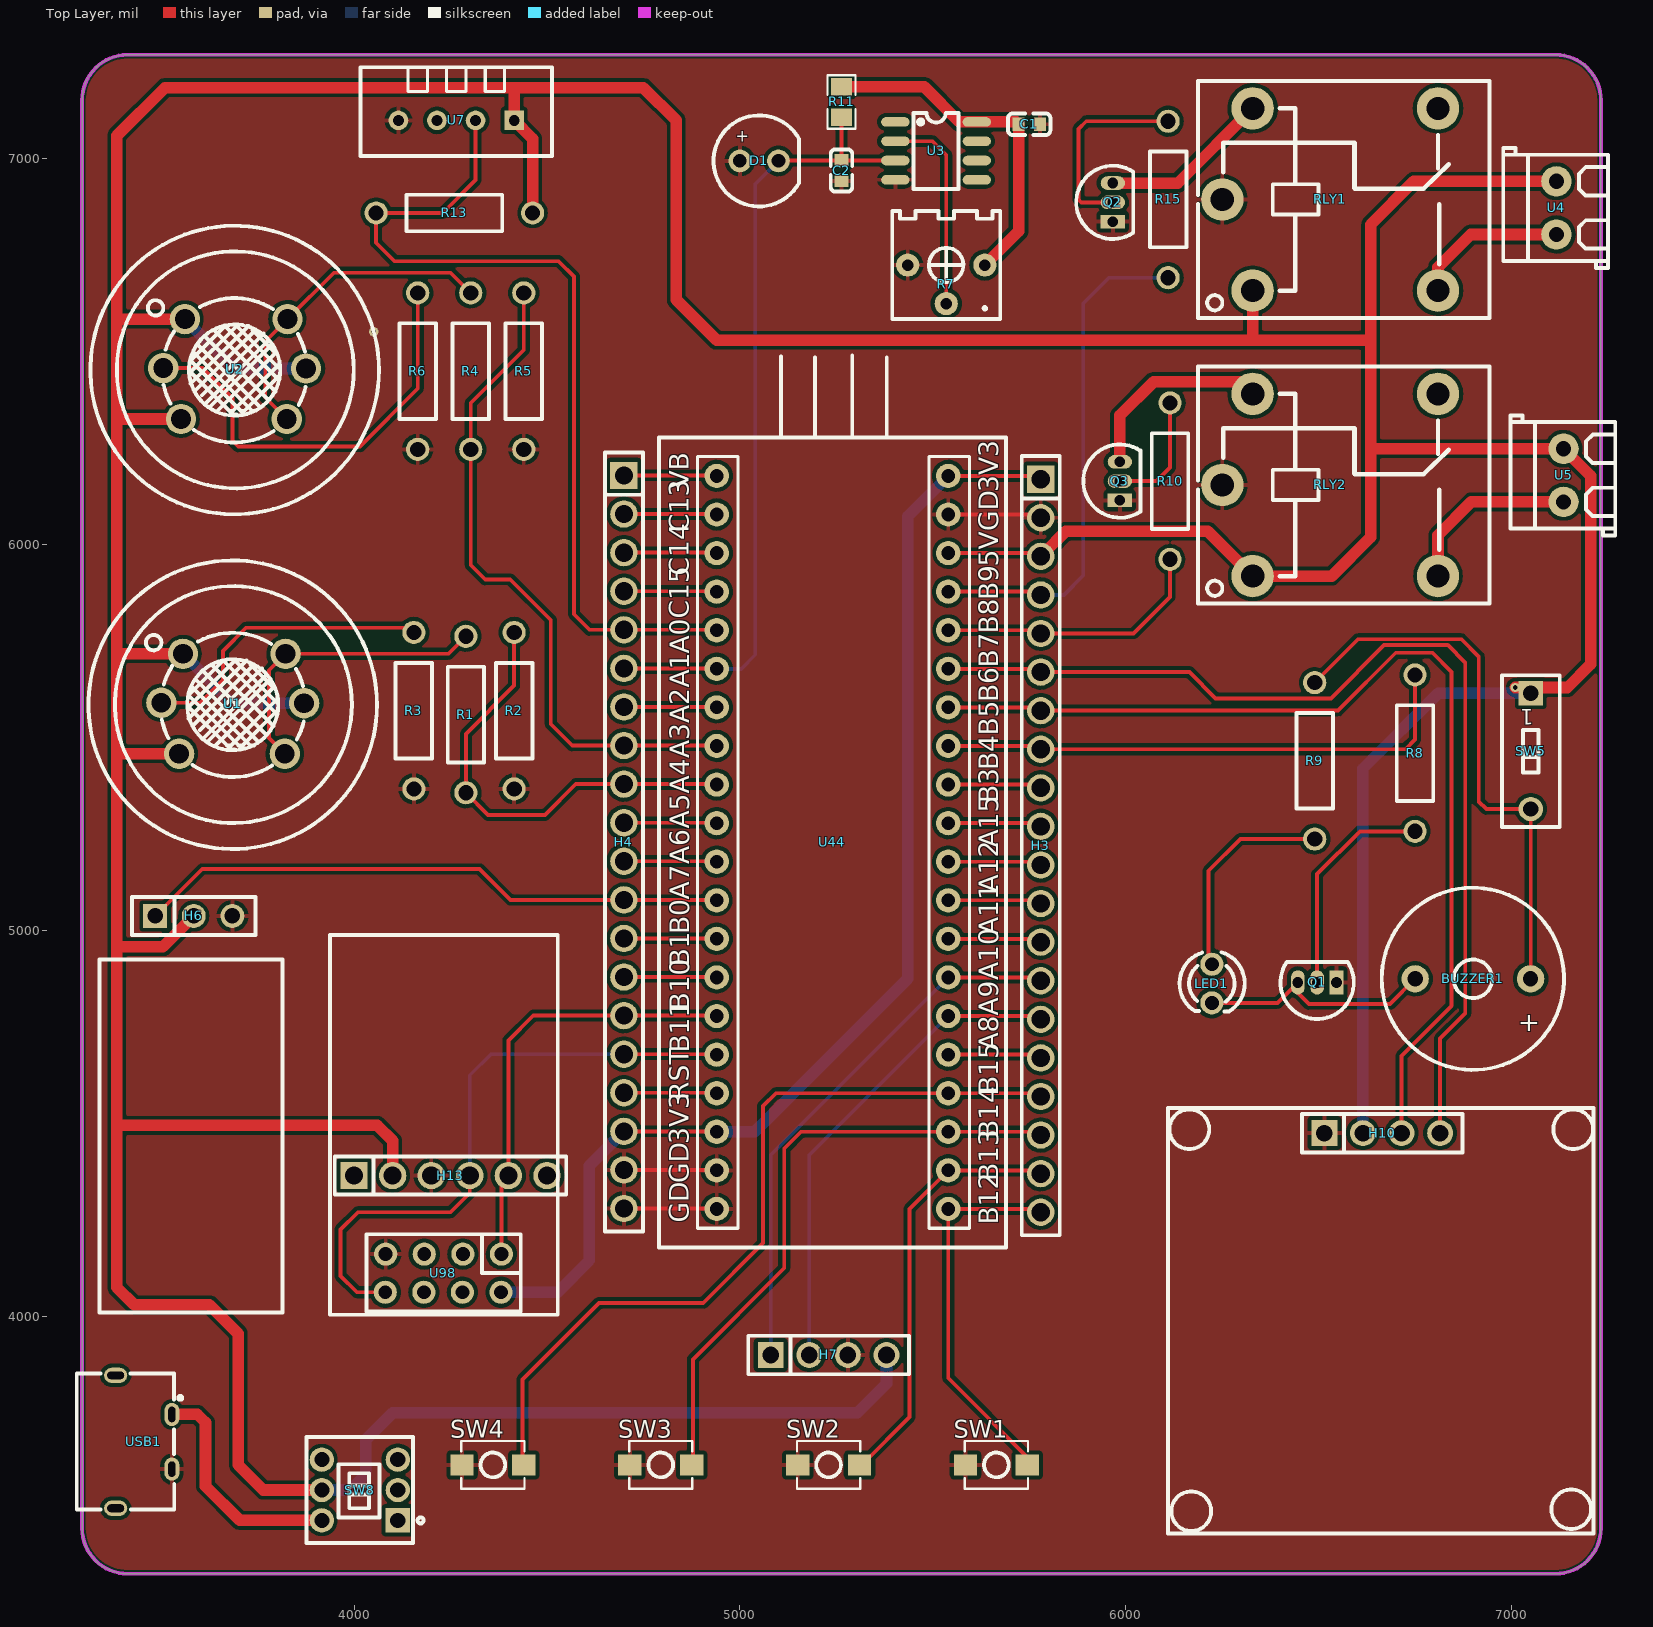
[diagram p0: Top Layer view]
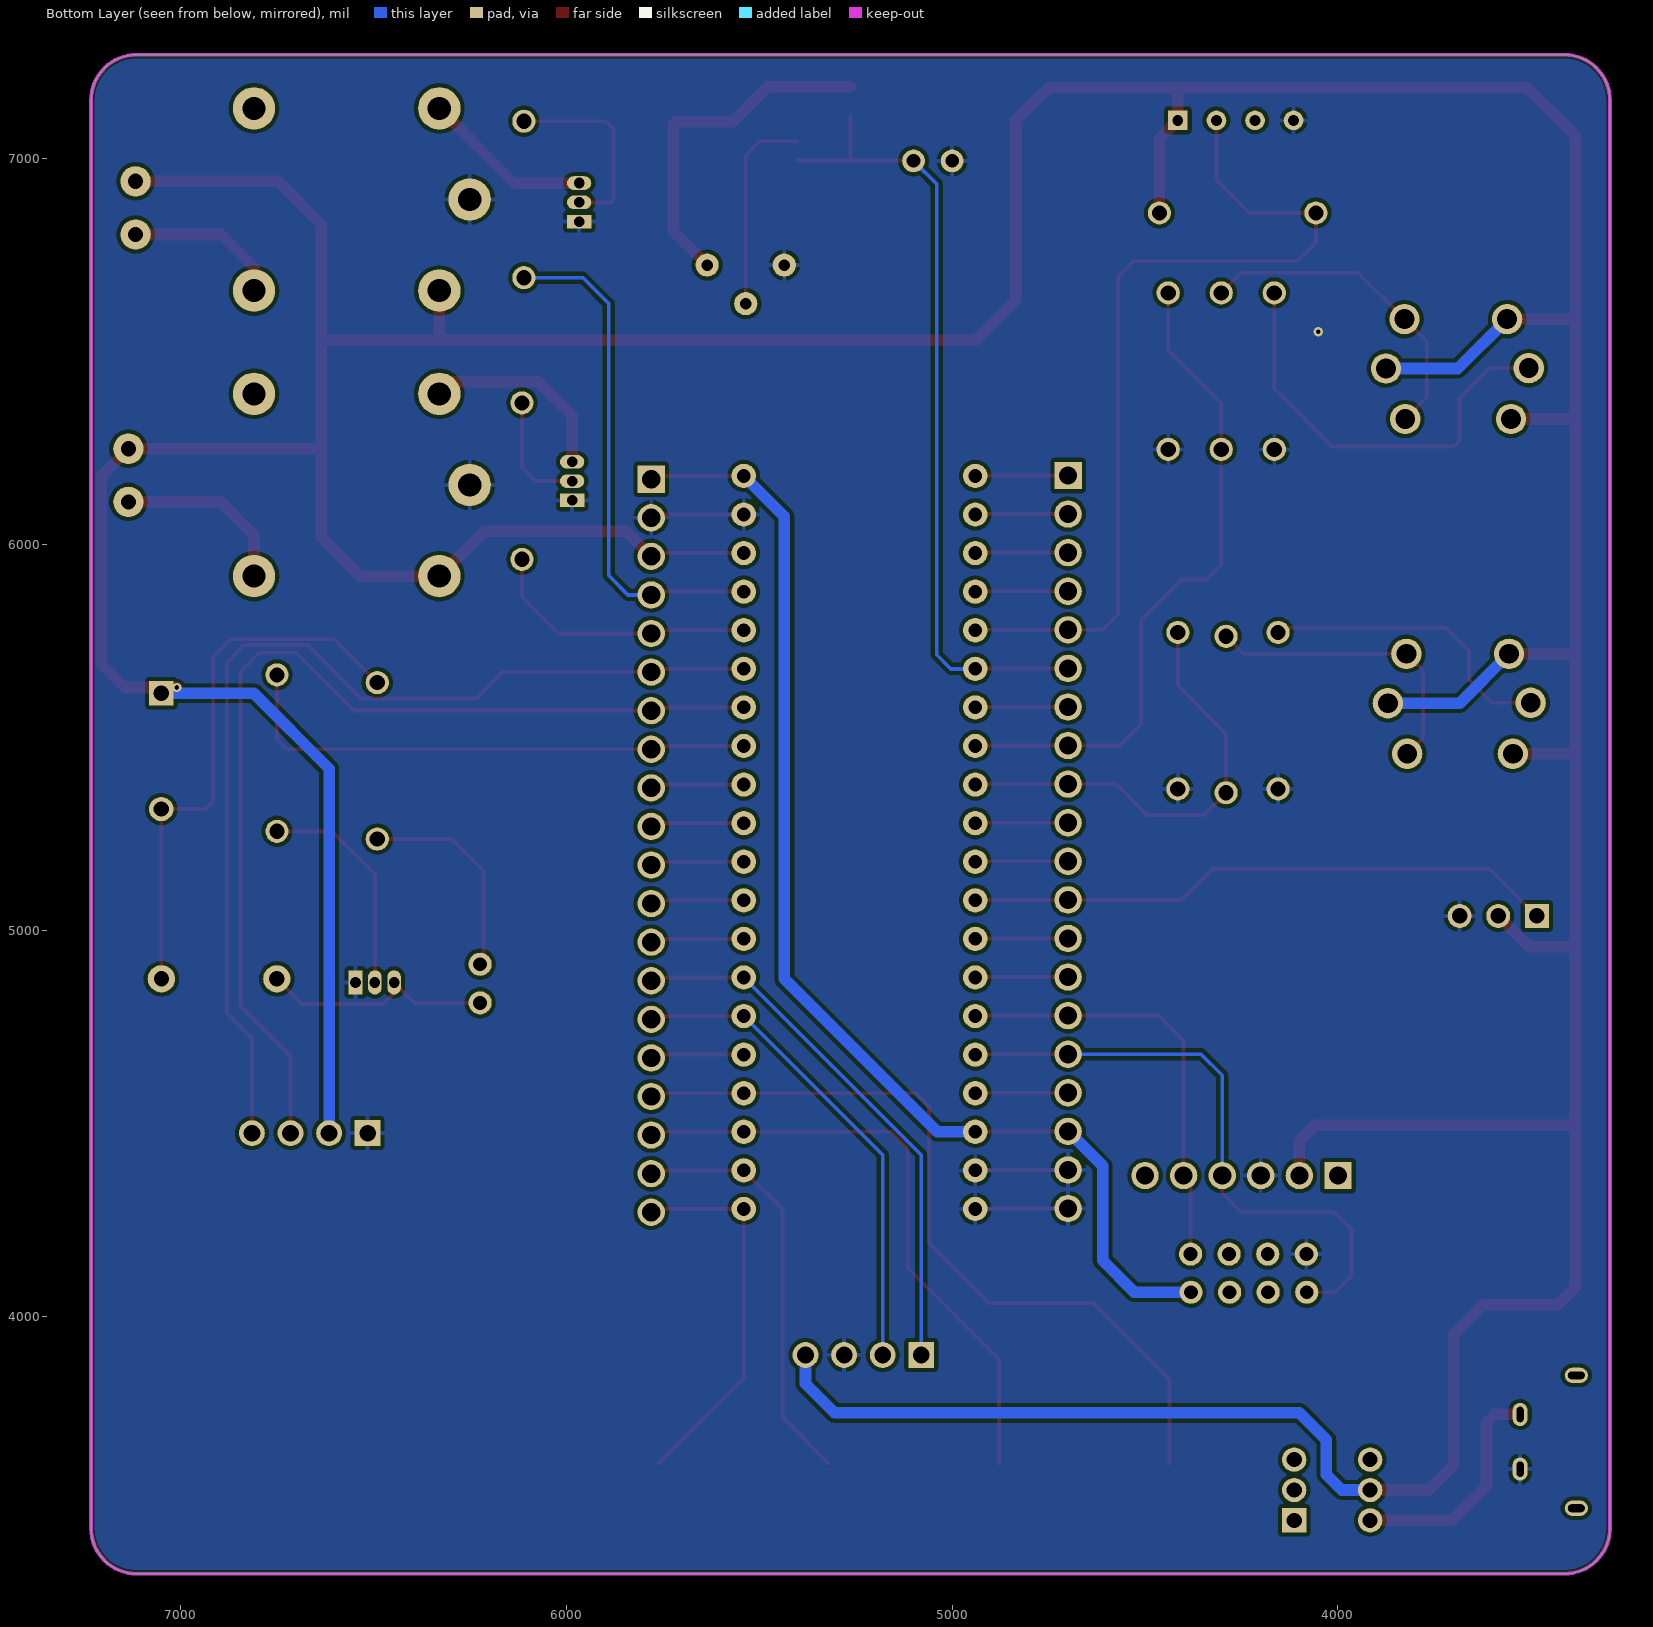
[diagram p1: Bottom Layer view, seen from below]
# Altium PCB MISC52003.pcbdoc
Units mil, origin at the board's own origin, x right, y up, seen from the top; angles counter-clockwise.
Board outline 3937.01 x 3937.01 mil, 2 copper layers (Top Layer, Bottom Layer), stack 62.206 mil thick; 44 components, 55 nets, 209 pads, 2 vias.

## Layer stack, top to bottom
Top Solder Mask Layer: solder mask 0.394, Dk 3.3
Top Layer: signal copper 1.379
Dielectric1: surface 59.449, FR4, Dk 4.5
Bottom Layer: signal copper 1.378
Bottom Solder Mask Layer: solder mask 0.394, Dk 3.3

## Board outline
3413.11,7270 ccw(c3413.11,7151.89) 3295,7151.89 3295,3451.1 ccw(c3413.11,3451.1) 3413.11,3332.99 7113.9,3332.99 ccw(c7113.9,3451.1) 7232.01,3451.1 7232.01,7151.89 ccw(c7113.9,7151.89) 7113.9,7270

## Design rules (kind name [scope] priority, off if disabled: settings)
BoardOutlineClearance copperThickness2oz_1 [All] p2 off: genericclearance=7.99 ignorepadtopadclearanceinfootprint=FALSE except(0: Arc-SplitContinuation Track-SplitContinuation SMDPad-SplitContinuation THPad-SplitContinuation Via-SplitContinuation Fill-SplitContinuation Region-SplitContinuation Poly-SplitContinuation Text-SplitContinuation Hole-SplitContinuation; 5.98: Arc-CutoutEdge SMDPad-CutoutEdge THPad-CutoutEdge Via-CutoutEdge Fill-CutoutEdge Region-CutoutEdge Text-CutoutEdge; 6.93: Hole-OutlineEdge Hole-CutoutEdge; 10: Poly-OutlineEdge Poly-CutoutEdge; 11.81: Arc-OutlineEdge Track-OutlineEdge SMDPad-OutlineEdge THPad-OutlineEdge Via-OutlineEdge Fill-OutlineEdge Region-OutlineEdge Text-OutlineEdge Track-CutoutEdge)
BoardOutlineClearance copperThickness1oz_1 [All] p4: genericclearance=4.02 ignorepadtopadclearanceinfootprint=FALSE except(0: Arc-SplitContinuation Track-SplitContinuation SMDPad-SplitContinuation THPad-SplitContinuation Via-SplitContinuation Fill-SplitContinuation Region-SplitContinuation Poly-SplitContinuation Text-SplitContinuation Hole-SplitContinuation; 6: SMDPad-CutoutEdge THPad-CutoutEdge Via-CutoutEdge Fill-CutoutEdge Region-CutoutEdge Text-CutoutEdge; 6.93: Hole-OutlineEdge Hole-CutoutEdge; 10: Poly-OutlineEdge Poly-CutoutEdge; 11.8: Arc-OutlineEdge Track-OutlineEdge SMDPad-OutlineEdge THPad-OutlineEdge Via-OutlineEdge Fill-OutlineEdge Region-OutlineEdge Text-OutlineEdge; 11.81: Arc-CutoutEdge Track-CutoutEdge)
Clearance copperThickness2oz [All] p1 off: gap=7.99 ignorepadtopadclearanceinfootprint=FALSE except(5.98: SMDPad-Track SMDPad-SMDPad THPad-Track SMDPad-THPad THPad-THPad Track-Via SMDPad-Via THPad-Via Via-Via Fill-Track Region-Track Fill-SMDPad Region-SMDPad Fill-THPad Region-THPad Fill-Via Region-Via Fill-Fill Fill-Region Region-Region Arc-Track Arc-SMDPad Arc-THPad Arc-Via Fill-Arc Region-Arc Arc-Arc Text-Track SMDPad-Text Text-THPad Text-Via Fill-Text Region-Text Arc-Text Text-Text; 6.93: Hole-Track Hole-SMDPad Hole-THPad Hole-Via Fill-Hole Region-Hole Hole-Arc Hole-Text; 10: Poly-Track Poly-SMDPad Poly-THPad Poly-Via Poly-Fill Poly-Region Poly-Poly Poly-Arc Poly-Text Poly-Hole)
Clearance copperThickness1oz [All] p3: gap=4.02 ignorepadtopadclearanceinfootprint=FALSE except(5.98: SMDPad-Track SMDPad-SMDPad THPad-Track SMDPad-THPad THPad-THPad Track-Via SMDPad-Via THPad-Via Via-Via Fill-Track Region-Track Fill-SMDPad Region-SMDPad Fill-THPad Region-THPad Fill-Via Region-Via Fill-Fill Fill-Region Region-Region; 6: Arc-Track Arc-SMDPad Arc-THPad Arc-Via Fill-Arc Region-Arc Arc-Arc Text-Track SMDPad-Text Text-THPad Text-Via Fill-Text Region-Text Arc-Text Text-Text; 6.93: Hole-Track Hole-SMDPad Hole-THPad Hole-Via Fill-Hole Region-Hole Hole-Arc Hole-Text; 10: Poly-Track Poly-SMDPad Poly-THPad Poly-Via Poly-Fill Poly-Region Poly-Poly Poly-Arc Poly-Text Poly-Hole)
Creepage creepage [All] p1: checkdistance=0 ignoreinternallayers=TRUE applytopolygonpour=TRUE
DiffPairsRouting differentialPair [All] p1: maxlimit=6 minlimit=6 mostfreqgap=6 toplayer_minwidth=5 toplayer_prefwidth=10 toplayer_maxwidth=100 toplayer_mingap=6 toplayer_prefgap=6 toplayer_maxgap=6 bottomlayer_minwidth=5 bottomlayer_prefwidth=10 bottomlayer_maxwidth=100 bottomlayer_mingap=6 bottomlayer_prefgap=6 bottomlayer_maxgap=6 maxuncoupledlength=10
HoleToHoleClearance otherClearance [All] p1: gap=11.81 allowstackedmicrovias=TRUE
Length netLength [All] p1: minlimit=0 maxlimit=0
MatchedLengths netLengthTolerance [All] p1: tolerance=1000
PasteMaskExpansion pasteMaskExpansion [All] p1: expansion=0
PlaneConnect innerPlane [All] p1: planeconnectstyle=Relief reliefexpansion=20 reliefentries=4 reliefconductorwidth=10 reliefairgap=10
PolygonConnect copperRegion [(InNet('GND'))] p1: connectstyle=Relief reliefconductorwidth=10 reliefentries=4 polygonreliefangle="90 Angle" airgapwidth=10 via.connectstyle=Relief via.reliefconductorwidth=10 via.reliefentries=4 via.polygonreliefangle="90 Angle" via.airgapwidth=10
RoutingVias viaSize [All] p1: holewidth=12.01 width=24.02 viastyle="Through Hole" minholewidth=11.81 minwidth=19.68 maxholewidth=248.03 maxwidth=393.7
SolderMaskExpansion solderMaskExpansion [IsVia] p1: expansion=-1000 istentingtop=TRUE
SolderMaskExpansion solderMaskExpansion [All] p2: expansion=2 istentingtop=FALSE
Width copperThickness2oz_2 [All] p1 off: maxlimit=100 minlimit=8 preferedwidth=10
Width copperThickness1oz_2 [All] p2: maxlimit=100 minlimit=5 preferedwidth=10

## Components (designator, comment, footprint, x,y, rotation, side; value= is the part's Value field where it differs from the comment)
BUZZER1 "2.3kHz" BUZ-TH_BD12.0-P7.60-D0.6-FD 6900,4875 r180 top
C1 "100nF" C0603 5750,7090 r180 top
C2 "100nF" C0603 5263.49,6970 r90 top
D1 "IR receiver" "IR 接收 D5" 5055,6995 r0 top
H3 "" HDR-TH_20P-P2.54-V-F 5780,5220 r270 top
H4 "" HDR-TH_20P-P2.54-V-F 4699.46,5229.58 r270 top
H6 "" HDR-TH_3P-P2.54-V-F 3584.58,5037.88 r0 top
H7 "" HDR-TH_4P-P2.54-V-F 5230,3900 r0 top
H10 "2.54-1*4P female" HDR-TH_4P-P2.54-V-F 6665,4475 r0 top
H13 "" HDR-TH_6P-P2.54-V-M-1 4250,4365 r0 top
LED1 "" LED_TH-3mm 6223.5,4862.73 r270 top
Q1 "" S8050_TO_92 6496.32,4865.58 r180 top
Q2 "" S8050_TO_92 5966.77,6887.54 r90 top
Q3 "" S8050_TO_92 5985,6165 r90 top
R1 "10kΩ" Res_1/4W 4290,5560 r90 top
R2 "10kΩ" Res_1/4W 4415,5570 r90 top
R3 "5Ω" Res_1/4W 4155,5570 r90 top
R4 "10kΩ" Res_1/4W 4302.5,6450 r90 top
R5 "10kΩ" Res_1/4W 4440,6450 r90 top
R6 "5Ω" Res_1/4W 4165,6450 r90 top
R7 "-" RES-ADJ-TH_3362P 5535,6675 r180 top
R8 "1kΩ" Res_1/4W 6750,5460 r270 top
R9 "120" Res_1/4W 6490,5440 r270 top
R10 "1kΩ" Res_1/4W 6115,6165 r90 top
R11 "10K" R0805 5263.49,7147.68 r90 top
R13 "10kΩ" Res_1/4W 4260,6860 r0 top
R15 "1kΩ" Res_1/4W 6110,6895 r90 top
RLY1 "SRD-05VDC-SL-C" RELAY-TH_SRD-XXVDC-XL-C 6530,6895 r0 top
RLY2 "SRD-05VDC-SL-C" RELAY-TH_SRD-XXVDC-XL-C 6530,6155 r0 top
SW1 "" Key_SMD_3x4x2 5665,3615 r0 top
SW2 "" Key_SMD_3x4x2 5230,3615 r0 top
SW3 "" Key_SMD_3x4x2 4795,3615 r0 top
SW4 "" Key_SMD_3x4x2 4360,3615 r0 top
SW5 "NDS-01V" SW-TH_2P-L3.9-W9.9-P2.54-LS7.6 7050,5465 r270 top
SW8 "TK-6700-1" SW-TH_TK-6700-1 4015,3550 r90 top
U1 "MQ-2" SENSOR-TH_MQ-2 3685.58,5587.88 r0 top
U2 "MQ-5" SENSOR-TH_MQ-2 3690.58,6455.41 r0 top
U3 "LM393" SOP-8_L4.9-W3.9-P1.27-LS6.0-BL 5508.69,7020.94 r270 top
U4 "KF350-3.5-2P" CONN-TH_P3.50_KF350-3.5-2P 7116.51,6873.11 r90 top
U5 "KF350-3.5-2P" CONN-TH_P3.50_KF350-3.5-2P 7135,6180 r90 top
U7 "DHT11" SENSOR-TH_DHT11 4265,7100 r180 top
U44 "" STM32最小系统板 5280,5485 r0 top
U98 "" WiFi封装 4230,4370 r0 top
USB1 "KH-TYPE-C-2P" USB-SMD_KH-TYPE-C-2P 3455,3675 r270 top

## Footprints (in the part's own frame and the unit in brackets; to place one, negate y for a bottom-side part, rotate by r counter-clockwise, add the part's x,y. Pads: shape width x height; smd on the part's side, far side on the other; paste and mask are expansions set on the pad)
BUZ-TH_BD12.0-P7.60-D0.6-FD [mm]
  round 1.8 hole 1 paste+0 mask+0.051: 1(-3.8,0) 2(3.8,0)
  silkscreen extent -6,-6 6,6
C0603 [mm]
  rect 0.8x0.9 smd: 1(-0.7,0) 2(0.7,0)
  silkscreen extent -1.39,-0.71 1.39,0.71
CONN-TH_P3.50_KF350-3.5-2P [mm]
  round 2 hole 1: 1(-1.75,0) 2(1.75,0)
  silkscreen extent -3.95,-3.4 3.95,3.5
HDR-TH_3P-P2.54-V-F [mil]
  rect 62x62 hole 40.16: 1(-100,0)
  round 62 hole 40.16: 2(0,0) 3(100,0)
  silkscreen extent -160,-49 160,49
HDR-TH_4P-P2.54-V-F [mm]
  rect 1.7x1.7 hole 1.1: 1(-3.81,0)
  round 1.7 hole 1.1: 2(-1.27,0) 3(1.27,0) 4(3.81,0)
  silkscreen extent -5.29,-1.27 5.29,1.27
HDR-TH_6P-P2.54-V-M-1 [mm]
  rect 1.8x1.8 hole 1.2: 1(-6.35,0)
  round 1.8 hole 1.2: 2(-3.81,0) 3(-1.27,0) 4(1.27,0) 5(3.81,0) 6(6.35,0)
  silkscreen extent -7.62,-1.25 7.62,1.25
HDR-TH_20P-P2.54-V-F [mm]
  rect 1.8x1.8 hole 1.2: 1(-24.13,0)
  round 1.8 hole 1.2: 2(-21.59,0) 3(-19.05,0) 4(-16.51,0) 5(-13.97,0) 6(-11.43,0) 7(-8.89,0) 8(-6.35,0) 9(-3.81,0) 10(-1.27,0) 11(1.27,0) 12(3.81,0) 13(6.35,0) 14(8.89,0) 15(11.43,0) 16(13.97,0) 17(16.51,0) 18(19.05,0) 19(21.59,0) 20(24.13,0)
  silkscreen extent -25.65,-1.25 25.65,1.25
"IR 接收 D5" [mm]
  round 1.5 hole 0.9 paste+0 mask+0.102: 1(-1.397,0) 2(1.143,0)
  silkscreen extent -3.12,-3 2.5,3
Key_SMD_3x4x2 [mm]
  rect 1.53x1.36 smd paste+0 mask+0.051: 1(-2.035,0) 2(2.035,0)
  silkscreen extent -2.08,-1.58 2.08,1.58
LED_TH-3mm [mil]
  round 60 hole 36 paste+0 mask+2: 1(-50,0) 2(50,0)
  silkscreen extent -81,-84 72,85
R0805 [mm]
  rect 1.133x1.377 smd paste-100 mask+0.051: 1(-1,0) 2(1,0)
  silkscreen extent -1.76,-0.92 1.76,0.92
RELAY-TH_SRD-XXVDC-XL-C [mil]
  round 110 hole 60: 1(-200.79,-236.22) 2(279.52,-236.2) 3(279.53,236.2) 4(-200.79,236.22) 5(-279.53,0)
  silkscreen extent -342,-307 413,307
RES-ADJ-TH_3362P [mil]
  round 60 hole 30: 1(-100,-50) 2(0,50) 3(100,-50)
  silkscreen extent -140,-190 140,90
Res_1/4W [mil]
  round 60 hole 39.37 paste+0 mask+2: 1(-202.76,0) 2(202.76,0)
  silkscreen extent -124,-47 124,47
S8050_TO_92 [mil]
  rect 35.4x63 hole 27.6 paste+0 mask+2: 1(-50,0)
  oval 35.4x63 hole 27.6 paste+0 mask+2: 2(0,0) 3(50,0)
  silkscreen extent -95,-53 95,95
SENSOR-TH_DHT11 [mil]
  rect 51x51 hole 28: 1(-150,0)
  round 51 hole 28: 2(-50,0) 3(50,0) 4(150,0)
  silkscreen extent -248,-138 248,93
SENSOR-TH_MQ-2 [mil]
  round 78.74 hole 51.18: 1(-129,129.5) 2(-185,2.5) 3(-139,-129.5) 4(135,-129.5) 5(185,1.5) 6(137,129.5)
  silkscreen extent -374,-376 374,371
SOP-8_L4.9-W3.9-P1.27-LS6.0-BL [mm]
  oval 0.63x1.865 smd: 1(-1.905,-2.682) 2(-0.635,-2.682) 3(0.635,-2.682) 4(1.905,-2.682) 5(1.905,2.682) 6(0.635,2.682) 7(-0.635,2.682) 8(-1.905,2.682)
  silkscreen extent -2.5,-1.5 2.5,1.48
STM32最小系统板 [mm]
  round 1.6 hole 0.9: 1(-8.634,17.614) 2(-8.634,15.074) 3(-8.634,12.534) 4(-8.634,9.994) 5(-8.634,7.454) 6(-8.634,4.914) 7(-8.634,2.374) 8(-8.634,-0.166) 9(-8.634,-2.706) 10(-8.634,-5.246) 11(-8.634,-7.786) 12(-8.634,-10.326) 13(-8.634,-12.866) 14(-8.634,-15.406) 15(-8.634,-17.946) 16(-8.634,-20.486) 17(-8.634,-23.026) 18(-8.634,-25.566) 19(-8.634,-28.106) 20(-8.634,-30.646) 21(6.606,17.614) 22(6.606,15.074) 23(6.606,12.534) 24(6.606,9.994) 25(6.606,7.454) 26(6.606,4.914) 27(6.606,2.374) 28(6.606,-0.166) 29(6.606,-2.706) 30(6.606,-5.246) 31(6.606,-7.786) 32(6.606,-10.326) 33(6.606,-12.866) 34(6.606,-15.406) 35(6.606,-17.946) 36(6.606,-20.486) 37(6.606,-23.026) 38(6.606,-25.566) 39(6.606,-28.106) 40(6.606,-30.646)
  silkscreen extent -12.44,-33.19 10.42,25.54
SW-TH_2P-L3.9-W9.9-P2.54-LS7.6 [mm]
  rect 1.6x1.6 hole 1 paste+0 mask+0.05: 1(-3.81,0)
  round 1.6 hole 1 paste+0 mask+0.05: 2(3.81,0)
  silkscreen extent -5,-1.91 5,1.91
SW-TH_TK-6700-1 [mm]
  rect 1.6x1.6 hole 1 paste+0 mask+0.051: 1(-2,-2.5)
  round 1.6 hole 1 paste+0 mask+0.051: 2(0,-2.5) 3(2,-2.5)
  round 1.6 hole 1 copper offset 0,0 paste+0 mask+0.051: 4(-2,2.5) 5(0,2.5) 6(2,2.5)
  silkscreen extent -3.5,-4.2 3.5,3.5
USB-SMD_KH-TYPE-C-2P [mm]
  oval 1.524x1 hole 0.45 slot 1 at 0 deg paste+0 mask+0.05: 1(-1.8,1.85) 2(1.8,1.85)
  oval 1x1.524 hole 0.5 slot 1.1 at 90 deg paste+0 mask+0.05: 3(4.375,-1.85) 4(-4.375,-1.85)
  silkscreen extent -4.5,-4.41 4.46,2.53
WiFi封装 [mil]
  round 60 hole 36: 1(152.01,-208.54) 2(150.91,-307.4) 3(52.01,-208.54) 4(50.91,-307.4) 5(-47.99,-208.54) 6(-49.09,-307.4) 7(-147.99,-208.54) 8(-149.09,-307.4)
  silkscreen extent -293,-366 298,618

## Via types
v1: diameter 24.02, hole 12, Top Layer to Bottom Layer, 2 vias

## Nets (pads, with @x,y where several pads share a name; then routed paths per layer and width w, separated by ;. In a path a pad name is that pad's centre, name@x,y a point inside that pad or via, vN(x,y) a via of type N, cw(c..) or ccw(c..) an arc to the next point about the centre after c; other vN are vias at no path point)
3V3: H3.1 H4.18 U44.18 U44.21 U98.2 | length 3136.5
  Top Layer w10: H4.18 U44.18@4940,4479.58 ; U44.21 H3.1@5795,6178.46
  Bottom Layer w30: U98.2 4527.6,4062.6 4610,4145 4610,4390.12 H4.18 ; U44.18 5038.46,4478.46 5435,4875 5435,6073.39 U44.21
$1N3: R1.2 U1.4 U1.6 | length 779.7
  Top Layer w10: U1.4 3780,5498.95 3780,5674.8 U1.6 4244.61,5717.38 R1.2
$1N5: R3.2 U1.2 | length 784
  Top Layer w10: U1.2 3600.38,5590.38 3660,5650 3660,5725 3720,5785 4142.76,5785 R3.2
$1N8: R6.2 U2.2 | length 1117.8
  Top Layer w10: U2.2 3607.09,6457.91 3685,6380 3685,6270 3700,6255 4015,6255 4165,6405 R6.2
$1N10: R4.2 U2.4 U2.6 | length 852.2
  Top Layer w10: U2.4 3770,6381.49 3770,6527.33 U2.6 3947.67,6705 4250.26,6705 R4.2
$1N88: BUZZER1.1 R9.1 SW5.2 | length 1448.6
  Top Layer w10: R9.1 6602.24,5755 6870,5755 6915,5710 6915,5335 6935,5315 SW5.2 7050,4875.4 BUZZER1.1
$1N89: BUZZER1.2 LED1.2 Q1.3 | length 614.5
  Top Layer w10: LED1.2 6393.47,4812.73 Q1.3 6446.32,4838.68 6475,4810 6685.4,4810 BUZZER1.2
$1N100: H4.17 U44.17 | length 240.5
  Top Layer w10: H4.17 U44.17@4940,4579.58
$1N103: H4.14 U44.14 | length 240.5
  Top Layer w10: H4.14 U44.14@4940,4879.58
$1N104: H4.13 U44.13 | length 240.5
  Top Layer w10: H4.13 U44.13@4940,4979.58
$1N106: H4.11 U44.11 | length 240.5
  Top Layer w10: H4.11 U44.11@4940,5179.58
$1N110: H4.7 U44.7 | length 240.5
  Top Layer w10: H4.7 U44.7@4940,5579.58
$1N113: H4.4 U44.4 | length 240.5
  Top Layer w10: H4.4 U44.4@4940,5879.58
$1N114: H4.3 U44.3 | length 240.5
  Top Layer w10: H4.3 U44.3@4940,5979.58
$1N115: H4.2 U44.2 | length 240.5
  Top Layer w10: H4.2 U44.2@4940,6079.58
$1N116: H4.1 U44.1 | length 240.5
  Top Layer w10: H4.1 U44.1@4940,6179.58
$1N125: H3.9 U44.29 | length 254.9
  Top Layer w10: U44.29 H3.9@5795,5378.46
$1N126: H3.10 U44.30 | length 254.9
  Top Layer w10: U44.30 H3.10@5795,5278.46
$1N127: H3.11 U44.31 | length 254.9
  Top Layer w10: U44.31 H3.11@5795,5178.46
$1N128: H3.12 U44.32 | length 254.9
  Top Layer w10: U44.32 H3.12@5795,5078.46
$1N129: H3.13 U44.33 | length 254.9
  Top Layer w10: U44.33 H3.13@5795,4978.46
$1N132: H3.16 U44.36 | length 254.9
  Top Layer w10: U44.36 H3.16@5795,4678.46
$1N154: RLY1.2 U4.1 | length 402.8
  Top Layer w30: RLY1.2 6809.53,6719.53 6894.21,6804.21 U4.1
$1N275: Q1.2 R8.2 | length 580.4
  Top Layer w10: Q1.2 6496.32,5146.32 6607.24,5257.24 R8.2
$1N288: Q2.2 R15.2 | length 515.4
  Top Layer w10: Q2.2 5885,6887.54 5877.93,6894.61 5877.93,7077.93 5897.76,7097.76 R15.2
$1N290: Q2.3 RLY1.4 | length 442.7
  Top Layer w30: Q2.3 6135.53,6937.54 RLY1.4
$1N291: Q3.3 RLY2.4 | length 513.6
  Top Layer w30: Q3.3 5985,6335.21 6072.38,6422.59 6297.84,6422.59 RLY2.4
$1N293: Q3.2 R10.2 | length 312.3
  Top Layer w10: Q3.2 6080,6165 6115,6200 R10.2
$1N298: RLY2.2 U5.1 | length 467.1
  Top Layer w30: RLY2.2 6809.53,6024.53 6896.1,6111.1 U5.1
$1N299: LED1.1 R9.2 | length 554.9
  Top Layer w10: LED1.1 6215,4921.24 6215,5155 6297.24,5237.24 R9.2
$1N302: R7.2 U3.2 | length 531.8
  Top Layer w10: U3.2 5499.06,7045.94 5535,7010 R7.2
+5V: H3.3 H6.2 H7.4 H10.2 H13.2 R13.2 RLY1.1 RLY2.1 SW5.1 SW8.5 U1.1 U1.3 U1.5 U2.1 U2.3 U2.5 U4.2 U5.2 U7.1 U44.23 | length 17757.5
  Top Layer w10: U44.23 H3.3@5788.46,5978.46
  Top Layer w30: 3385.03,5717.38 U1.1 ; U1.3 3388.56,5458.38 3385,5461.93 ; U2.3 3388.18,6325.91 3385,6329.09 ; U2.1 3387.29,6584.91 3385,6587.2 ; H6.2 3504.66,4957.95 3385,4957.95 ; SW8.5 3765,3550 3700,3615 3700,3955 3625,4030 3430,4030 3385,4075 3385,4490.1 ; H13.2 4100,4455 4060,4495 3389.9,4495 3385,4490.1 ; R13.2 4462.76,7052.24 U7.1 4415,7183.35 4416.65,7185 ; H3.3 5788.46,5978.46 5845,6035 6212.99,6035 RLY2.1 6533.78,5918.78 6635,6020 6635,6254.11 ; RLY1.1 6329.21,6530.46 6328.75,6530 ; v1(7010,5630) 7145,5630 7205,5690 7205,6178.9 U5.2 6640.22,6248.9 6635,6254.11 ; U4.2 6747,6942 6635,6830 6635,6530 ; 3385,4490.1 3385,4957.95 ; 3385,4957.95 3385,5461.93 ; 3385,5461.93 3385,5717.41 3385,6329.09 ; 3385,6329.09 3385,6587.2 ; 3385,6587.2 3385,7060 3510,7185 4416.65,7185 ; 4416.65,7185 4750,7185 4835,7100 4835,6635 4940,6530 6328.75,6530 ; 6328.75,6530 6635,6530 ; 6635,6254.11 6635,6530
  Bottom Layer w30: U1.1 3684.58,5589.38 U1.5 ; U2.1 3689.58,6456.91 U2.5 ; SW8.5 3990,3550 4030,3590 4030,3680 4100,3750 5305,3750 5380,3825 H7.4 ; H10.2 6615,5420 6810,5615 SW5.1
DO: U3.1
GND: C1.1 C2.1 D1.1 H3.2 H4.19 H4.20 H6.3 H7.3 H10.1 H13.3 Q1.1 Q2.1 Q3.1 R2.1 R3.1 R5.1 R6.1 R7.3 RLY1.5 RLY2.5 SW1.1 SW2.1 SW3.1 SW4.1 U3.4 U7.4 U44.19 U44.20 U44.22 U98.7 USB1.2 | length 736
  Top Layer w10: H4.20 U44.20@4940,4279.58 ; H4.19 U44.19@4940,4379.58 ; U44.22 H3.2@5795,6078.46
  other v1: 4051.2,6552.12
PA0: H4.5 R13.1 U7.2 U44.5 | length 2336.1
  Top Layer w10: U7.2 4315,6945 4230,6860 R13.1 4057.24,6782.76 4105,6735 4530,6735 4570,6695 4570,5820 4610.42,5779.58 H4.5 U44.5@4940,5779.58
PA1: C2.2 D1.2 H4.6 R11.1 U3.3 U44.6 | length 2074.7
  Top Layer w10: H4.6 U44.6@4940,5679.58 ; D1.2 5100.94,6995.94 U3.3 ; C2.2 R11.1
  Bottom Layer w10: U44.6 5003.46,5678.46 5040,5715 5040,6935 D1.2
PA3: H4.8 R4.1 R5.2 U44.8 | length 1751.7
  Top Layer w10: R5.2 4440,6505 4302.5,6367.5 R4.1 4302.5,5947.5 4340,5910 4405,5910 4510,5805 4510,5535 4565.42,5479.58 H4.8 U44.8@4940,5479.58
PA4: H4.9 R1.1 R2.2 U44.9 | length 1174
  Top Layer w10: R2.2 4415,5635 4290,5510 R1.1 4347.24,5300 4495,5300 4574.58,5379.58 H4.9 U44.9@4940,5379.58
PA5: H4.10 U44.10 | length 240.5
  Top Layer w10: H4.10 U44.10@4940,5279.58
PA7: H4.12 H6.1 U44.12 | length 1539.3
  Top Layer w10: H6.1 3606.7,5160 4325,5160 4405.42,5079.58 H4.12 U44.12@4940,5079.58
PB5: H3.8 R8.1 U44.28 | length 1403
  Top Layer w10: U44.28 H3.8@5795,5478.46 ; H3.8 6725,5470 6750,5495 R8.1
PB6: H3.7 H10.3 U44.27 | length 2651.6
  Top Layer w10: U44.27 H3.7@5795,5578.46 ; H3.7 6550,5570 6700,5720 6795,5720 6845,5670 6845,4805 6715,4675 H10.3
PB7: H3.6 H10.4 U44.26 | length 2706
  Top Layer w10: U44.26 H3.6@5795,5678.46 ; H3.6 6165,5670 6233.22,5601.78 6531.78,5601.78 6670,5740 6835,5740 6880,5695 6880,4785 6815,4720 H10.4
PB8: H3.5 R10.1 U44.25 | length 726.5
  Top Layer w10: U44.25 H3.5@5795,5778.46 ; H3.5 6020,5770 6115,5865 R10.1
PB9: H3.4 R15.1 U44.24 | length 1338.5
  Top Layer w10: U44.24 H3.4@5795,5878.46
  Bottom Layer w10: H3.4 5840,5870 5890,5920 5890,6625 5957.24,6692.24 R15.1
PB12: H3.20 SW1.2 U44.40 | length 1006.1
  Top Layer w10: SW1.2@5761.51,3618.99 5540.08,3840.43 U44.40 H3.20@5795,4278.46
PB13: H3.19 SW2.2 U44.39 | length 1105.6
  Top Layer w10: SW2.2@5319.85,3618.99 5440,3739.14 5440,4278.39 U44.39 H3.19@5795,4378.46
PB14: H3.18 SW3.2 U44.38 | length 1612.1
  Top Layer w10: SW3.2@4878.18,3618.99 4878.18,3888.18 5115,4125 5115,4435 5158.46,4478.46 U44.38 H3.18@5795,4478.46
PB15: H3.17 SW4.2 U44.37 | length 2091.3
  Top Layer w10: SW4.2@4436.51,3618.99 4436.51,3836.51 4635,4035 4905,4035 5060,4190 5060,4545 5093.46,4578.46 U44.37 H3.17@5795,4578.46
U1_RX: H3.14 H7.1 U44.34 | length 1424
  Top Layer w10: U44.34 H3.14@5795,4878.46
  Bottom Layer w10: H7.1 5080,4418.39 U44.34
U1_TX: H3.15 H7.2 U44.35 | length 1282.5
  Top Layer w10: U44.35 H3.15@5795,4778.46
  Bottom Layer w10: H7.2 5180,4418.39 U44.35
U3_RX: H4.16 H13.4 U44.16 U98.8 | length 1595.4
  Top Layer w10: U98.8 4007.4,4062.6 3965,4105 3965,4225 4010,4270 4250,4270 4300,4320 H13.4 ; H4.16 U44.16@4940,4679.58
  Bottom Layer w10: H13.4 4300,4625 4354.58,4679.58 H4.16
U3_TX: H4.15 H13.5 U44.15 U98.1 | length 1127.7
  Top Layer w10: U98.1 4382.01,4347.01 H13.5 4400,4715 4464.58,4779.58 H4.15 U44.15@4940,4779.58
VCC: C1.2 R7.1 R11.2 U3.8 | length 900.4
  Top Layer w30: R11.2 5477.95,7187.05 5569.06,7095.94 U3.8 5716.5,7095.94 C1.2 5722.44,6812.44 R7.1
VUSB: SW8.4 USB1.1 | length 599.1
  Top Layer w30: USB1.1 3594.13,3745.87 3615,3725 3615,3560 3703.74,3471.26 SW8.4
pads on no net: H13.1 H13.6 RLY1.3 RLY2.3 SW8.1 SW8.2 SW8.3 SW8.6 U3.5 U3.6 U3.7 U7.3 U98.3 U98.4 U98.5 U98.6 USB1.3 USB1.4

## Polygon pours and split planes (outlines as drawn)
GND on Bottom Layer (solid, remove dead copper, pour order 2): 3000,7550 3000,3000 7640,3000 7640,7550
GND on Top Layer (solid, remove dead copper, pour order 0): 3110,7440 3110,3130 7615,3130 7615,7440

## Keep-outs
Board Outline Layer:
  the board outline again, w10

## Silkscreen, mask and mechanical layers (free items; w line width, h text height)
Top Silkscreen Layer:
  lines w10: 3340,4010 3340,4925 3815,4925 3815,4010 3340,4010